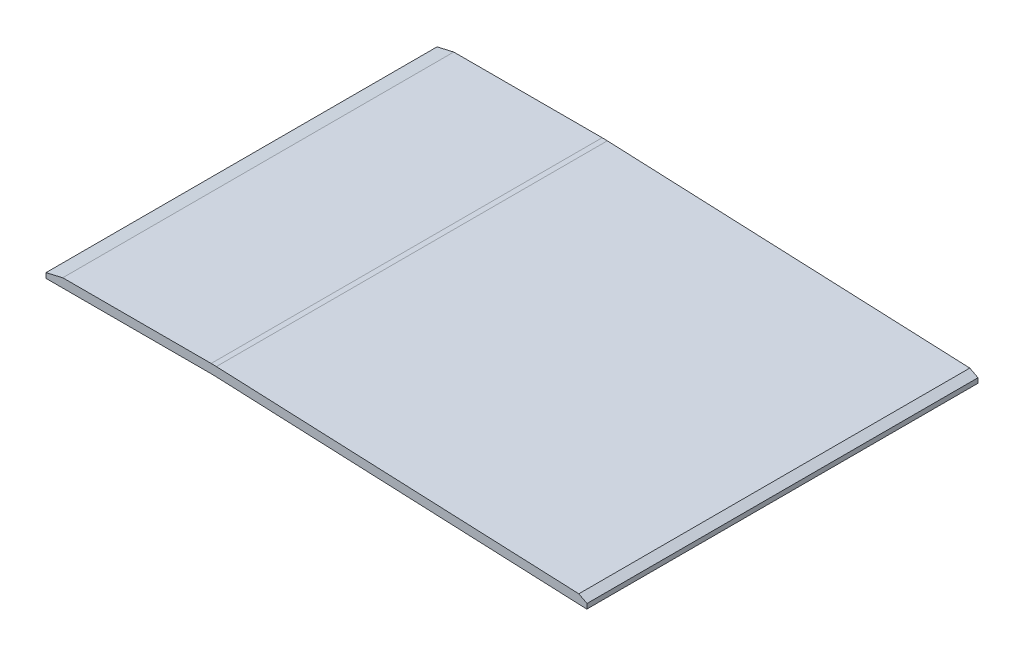
from build123d import *

# Parameters (mm, degrees)
BOSS_EXTRUDE1_DEPTH = 700


with BuildPart() as part:
    # Sketch1 → Boss-Extrude1 (new body)
    with BuildSketch(Plane.XY):
        with BuildLine():
            Line((0, 0), (295.706857871, 0))
            ThreePointArc((295.706857871, 0), (299.999011252, -0.046061756), (304.289187591, -0.184225806))
            Line((304.289187591, -0.184225806), (968.2, -28.7))
            Line((968.2, -28.7), (968.586204837, -19.708290161))
            Line((968.586204837, -19.708290161), (953.900403313, -12.071063335))
            Line((953.900403313, -12.071063335), (304.975773969, 15.801036129))
            ThreePointArc((304.975773969, 15.801036129), (300.342383522, 15.950253304), (295.706857871, 16))
            Line((295.706857871, 16), (30, 16))
            Line((30, 16), (0, 9))
            Line((0, 9), (0, 0))
        make_face()
    extrude(amount=BOSS_EXTRUDE1_DEPTH)


solid = part.part
